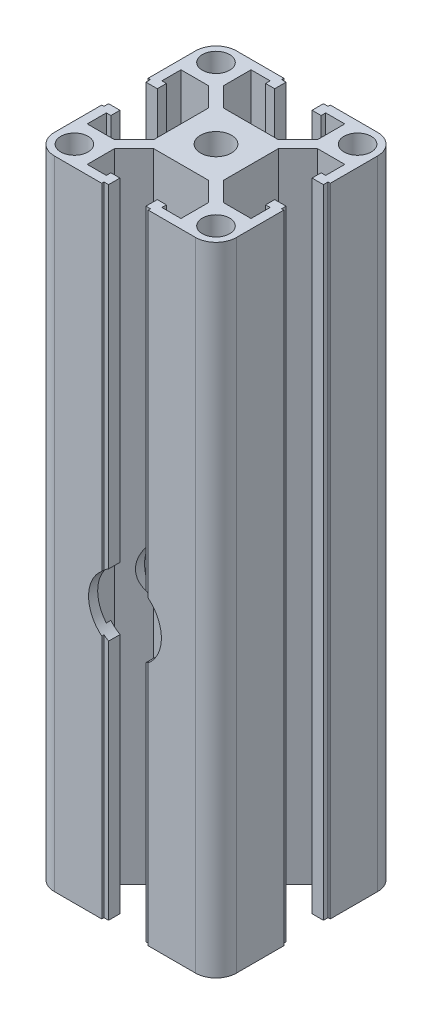
SolidWorks part; units mm, degrees
ref_plane "主视基准图" through (0, 0, 0) normal (0, 0, 1) x (1, 0, 0)
ref_plane "上视基准图" through (0, 0, 0) normal (0, 1, 0) x (1, 0, 0)
ref_plane "右视基准图" through (0, 0, 0) normal (1, 0, 0) x (0, 0, -1)
sketch "草图1" plane through (0, 0, 0) normal (0, 0, 1) x (1, 0, 0)
  line L0 (0, 0) -> (0, 140)
  dimension "D1" = 140
other "结构构件1"
ref_plane "基准面1" through (0, 0, 0) normal (0, 1, 0) x (-1, 0, 0)
sketch "Sketch16" plane through (0, 0, 0) normal (0, 1, 0) x (-1, 0, 0)
  line L0 (-5.1, 20) -> (-5.1, 19.5)
  line L1 (-5.1, 19.5) -> (-4.1, 19.5)
  line L2 (-4.1, 19.5) -> (-4.1, 17)
  line L3 (-6.1, 18) -> (-10.3, 18)
  line L4 (-15.5, -20) -> (-5.1, -20)
  line L5 (-20, -15.5) -> (-20, -5.1)
  line L6 (15.5, 20) -> (5.1, 20)
  line L7 (20, 15.5) -> (20, 5.1)
  line L8 (0, 14.8756) -> (0, 0) construction
  line L9 (0, 0) -> (14.1675, 0) construction
  line L10 (-10.3, 18) -> (-10.3, 12)
  line L11 (-10.3, 12) -> (-6, 7.7)
  line L12 (-6, 7.7) -> (6, 7.7)
  line L13 (10.3, 12) -> (6, 7.7)
  line L14 (10.3, 18) -> (10.3, 12)
  line L15 (6.1, 18) -> (10.3, 18)
  line L16 (4.1, 19.5) -> (4.1, 17)
  line L17 (5.1, 19.5) -> (4.1, 19.5)
  line L18 (5.1, 20) -> (5.1, 19.5)
  line L19 (-5.1, 20) -> (-15.5, 20)
  line L20 (20, 5.1) -> (19.5, 5.1)
  line L21 (0, 0) -> (-15.5563, 15.5563) construction
  line L22 (0, 0) -> (-15.5563, -15.5563) construction
  line L25 (19.5, 5.1) -> (19.5, 4.1)
  line L26 (19.5, 4.1) -> (17, 4.1)
  line L27 (17, 6.1) -> (17, 4.1)
  line L28 (18, 6.1) -> (17, 6.1)
  line L29 (18, 6.1) -> (18, 10.3)
  line L30 (18, 10.3) -> (12, 10.3)
  line L31 (12, 10.3) -> (7.7, 6)
  line L32 (7.7, 6) -> (7.7, -6)
  line L33 (12, -10.3) -> (7.7, -6)
  line L34 (18, -10.3) -> (12, -10.3)
  line L35 (18, -6.1) -> (18, -10.3)
  line L36 (18, -6.1) -> (17, -6.1)
  line L37 (17, -4.1) -> (17, -6.1)
  line L38 (19.5, -4.1) -> (17, -4.1)
  line L39 (19.5, -5.1) -> (19.5, -4.1)
  line L40 (20, -5.1) -> (19.5, -5.1)
  line L41 (5.1, -20) -> (5.1, -19.5)
  line L42 (5.1, -19.5) -> (4.1, -19.5)
  line L43 (4.1, -19.5) -> (4.1, -17)
  line L44 (6.1, -17) -> (4.1, -17)
  line L45 (6.1, -18) -> (6.1, -17)
  line L46 (6.1, -18) -> (10.3, -18)
  line L47 (10.3, -18) -> (10.3, -12)
  line L48 (10.3, -12) -> (6, -7.7)
  line L49 (6, -7.7) -> (-6, -7.7)
  line L50 (-10.3, -12) -> (-6, -7.7)
  line L51 (-10.3, -18) -> (-10.3, -12)
  line L52 (-6.1, -18) -> (-10.3, -18)
  line L53 (-6.1, -18) -> (-6.1, -17)
  line L54 (-4.1, -17) -> (-6.1, -17)
  line L55 (-4.1, -19.5) -> (-4.1, -17)
  line L56 (-5.1, -19.5) -> (-4.1, -19.5)
  line L57 (-5.1, -20) -> (-5.1, -19.5)
  line L58 (-20, -5.1) -> (-19.5, -5.1)
  line L59 (5.1, -20) -> (15.5, -20)
  line L60 (-20, 5.1) -> (-20, 15.5)
  line L61 (-19.5, -5.1) -> (-19.5, -4.1)
  line L62 (-6.1, 18) -> (-6.1, 17)
  line L63 (-6.1, 17) -> (-4.1, 17)
  line L64 (6.1, 18) -> (6.1, 17)
  line L65 (4.1, 17) -> (6.1, 17)
  line L66 (-19.5, -4.1) -> (-17, -4.1)
  line L71 (-17, -6.1) -> (-17, -4.1)
  line L72 (-18, -6.1) -> (-17, -6.1)
  line L73 (-18, -6.1) -> (-18, -10.3)
  line L74 (-18, -10.3) -> (-12, -10.3)
  line L75 (-12, -10.3) -> (-7.7, -6)
  line L76 (-7.7, -6) -> (-7.7, 6)
  line L77 (-12, 10.3) -> (-7.7, 6)
  line L78 (-18, 10.3) -> (-12, 10.3)
  line L79 (-18, 6.1) -> (-18, 10.3)
  line L80 (-18, 6.1) -> (-17, 6.1)
  line L81 (-17, 4.1) -> (-17, 6.1)
  line L82 (-19.5, 4.1) -> (-17, 4.1)
  line L83 (-19.5, 5.1) -> (-19.5, 4.1)
  line L84 (-20, 5.1) -> (-19.5, 5.1)
  line L85 (20, -5.1) -> (20, -15.5)
  circle A0 centre (0, 0) radius 3.4
  arc A1 (-20, 15.5) -> (-15.5, 20) centre (-15.5, 15.5) cw
  arc A2 (20, 15.5) -> (15.5, 20) centre (15.5, 15.5) ccw
  arc A3 (-15.5, -20) -> (-20, -15.5) centre (-15.5, -15.5) cw
  arc A4 (15.5, -20) -> (20, -15.5) centre (15.5, -15.5) ccw
  circle A5 centre (-15.5563, 15.5563) radius 3
  circle A6 centre (15.5563, 15.5563) radius 3
  circle A7 centre (15.5563, -15.5563) radius 3
  circle A8 centre (-15.5563, -15.5563) radius 3
  point P2 (0, 10)
  point P3 (0, 0)
  point P4 (0, 0)
  point P5 (-20, -20)
  point P6 (20, -20)
  point P7 (20, 20)
  point P8 (-20, 20)
  point P36 (-20, 20)
  point P39 (20, 20)
  dimension "D1" = 20.6
  dimension "D2" = 40
  dimension "D3" = 8.2
  dimension "D4" = 10.2
  dimension "D5" = 12.3
  dimension "D6" = 6.8
  dimension "D7" = 4.5
  dimension "D8" = 45
  dimension "D12" = 6
  dimension "D13" = 22
  dimension "D9" = 0.5
  dimension "D10" = 2
  dimension "D11" = 12
  dimension "D16" = 3
  dimension "D17" = 2
hole_wizard "M8 六角凹头螺钉的柱形沉头孔1" positions "草图5" profile "草图4" counterbore size "M8" standard "Iso" end condition through all
sketch "草图5" plane through (9.5819, -44.0931, 20) normal (0, 0, -1) x (-1, 0, 0)
  line L0 (20, 114.0931) -> (-5.9181, 114.0931) construction
  line L2 (-5.9181, 184.0931) -> (-5.9181, 44.0931) construction
  line L6 (9.5819, 44.0931) -> (9.5819, 270.5931) construction
  line L7 (4.4819, 44.0931) -> (-5.9181, 44.0931) construction
  point P0 (9.5819, 104.0931)
  dimension "D1" = 60
sketch "草图4" plane through (0, 60, 20) normal (1, 0, 0) x (0, -1, 0)
  line L0 (0, 0) -> (0, 40)
  line L1 (0, 40) -> (4.5, 40)
  line L3 (4.5, 40) -> (4.5, 12.3)
  line L4 (4.5, 12.3) -> (8, 12.3)
  line L5 (8, 12.3) -> (8, 0)
  line L7 (8, 0) -> (0, 0)
  line L11 (0, -6.35) -> (0, 107.95) construction
  dimension "通孔孔直径" = 9
  dimension "通孔孔深度" = 40
  dimension "柱形沉头孔直径" = 16
  dimension "柱形沉头孔深度" = 12.3
